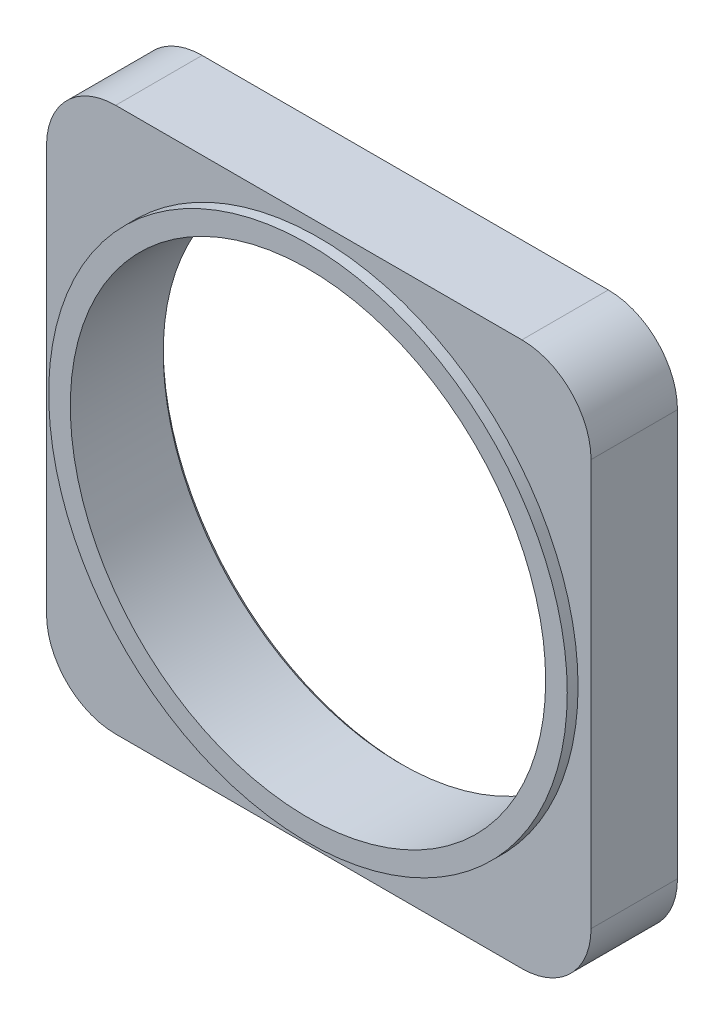
SolidWorks part; units mm, degrees
ref_plane "Front Plane" through (0, 0, 0) normal (0, 0, 1) x (1, 0, 0)
ref_plane "Top Plane" through (0, 0, 0) normal (0, 1, 0) x (1, 0, 0)
ref_plane "Right Plane" through (0, 0, 0) normal (1, 0, 0) x (0, 0, -1)
sketch "Sketch1" plane through (0, 0, 0) normal (0, 0, 1) x (1, 0, 0)
  line L0 (16, 0) -> (110, 0)
  line L1 (126, 16) -> (126, 110)
  line L2 (110, 126) -> (16, 126)
  line L3 (0, 110) -> (0, 16)
  circle A0 centre (63, 63) radius 55
  arc A1 (0, 16) -> (16, 0) centre (16, 16) ccw
  arc A2 (126, 16) -> (110, 0) centre (110, 16) cw
  arc A3 (126, 110) -> (110, 126) centre (110, 110) ccw
  arc A4 (0, 110) -> (16, 126) centre (16, 110) cw
  point P9 (0, 0)
  dimension "D1" = 16
extrude "Boss-Extrude1" add sketch "Sketch1" along normal blind 20
sketch "Sketch2" plane through (0, 0, 20) normal (0, 0, 1) x (1, 0, 0)
  circle A0 centre (63, 63) radius 60
  circle A1 centre (63, 63) radius 55
extrude "Boss-Extrude2" add sketch "Sketch2" along normal blind 2.5
sketch "Sketch3" plane through (0, 0, 0) normal (0, 0, -1) x (-1, 0, 0)
  circle A4 centre (-16, 110) radius 4.25
  circle A5 centre (-110, 110) radius 4.25
  circle A6 centre (-16, 16) radius 4.25
  circle A7 centre (-110, 16) radius 4.25
hole_wizard "M10x1.5 Tapped Hole1" positions "3DSketch1" profile "Sketch4" tap size "M10x1.5" standard "Ansi Metric"
sketch3d "3DSketch1"
  point P0 (110, 110, 0)
  point P3 (16, 110, 0)
  point P6 (16, 16, 0)
  point P9 (110, 16, 0)
sketch "Sketch4" plane through (110, 110, 0) normal (1, 0, 0) x (0, 1, 0)
  line L0 (0, 0) -> (0, 14.5537)
  line L1 (0, 14.5537) -> (4.25, 12)
  line L2 (4.25, 12) -> (4.25, 0)
  line L5 (4.25, 0) -> (0, 0)
  line L10 (0, 14.5537) -> (-4.25, 12) construction
  line L11 (0, -6.35) -> (0, 107.95) construction
  dimension "螺纹孔钻头直径" = 8.5
  dimension "螺纹孔钻头深度" = 12
  dimension "导头角度" = 118
cosmetic thread "Cosmetic thread 1" parameters "D1"=10, "D2"=10
cosmetic thread "Cosmetic thread 2" parameters "D1"=10, "D2"=10
cosmetic thread "Cosmetic thread 3" parameters "D1"=10, "D2"=10
cosmetic thread "Cosmetic thread 4" parameters "D1"=10, "D2"=10
chamfer "Chamfer1" distance 1 angle 45 1 edges at (118, 63, 0)
